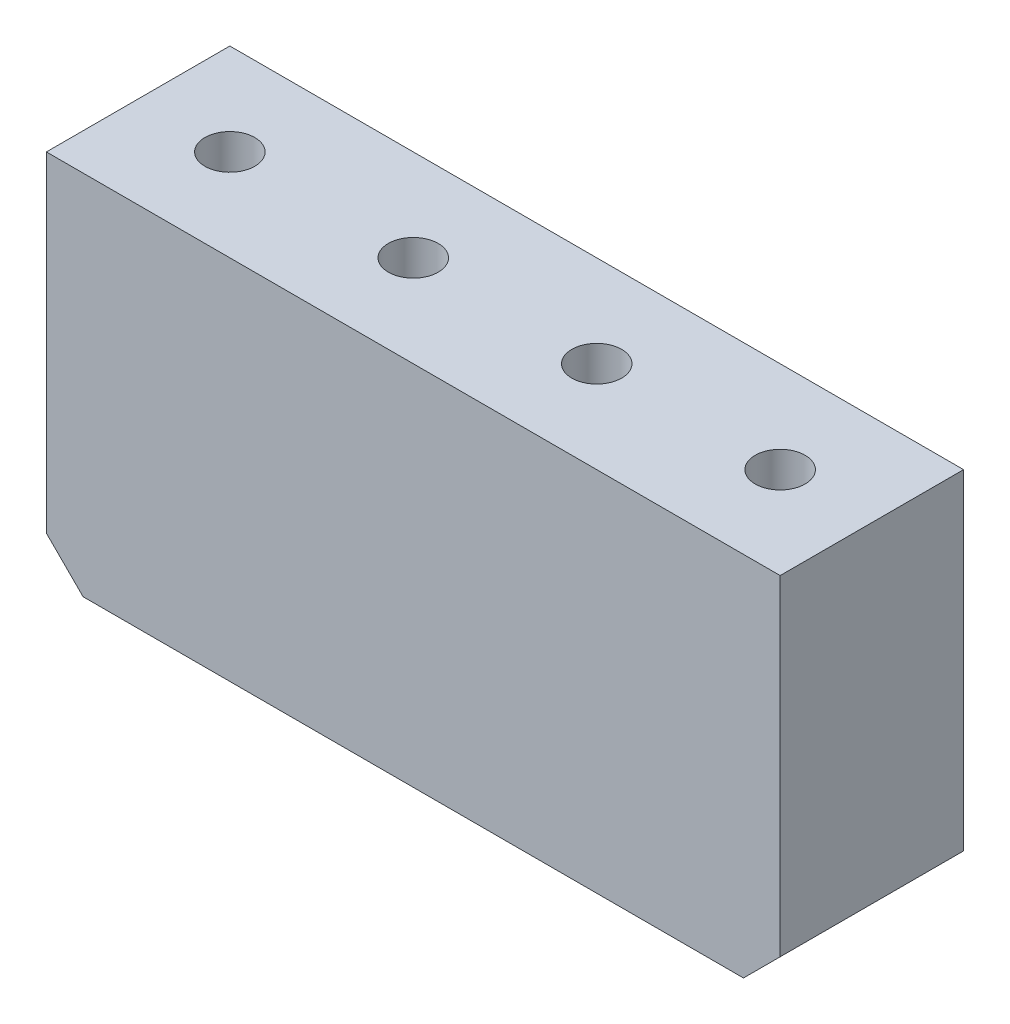
from build123d import *

# Parameters (mm, degrees)
SKETCH1_W           = 100
SKETCH1_H           = 50
BOSS_EXTRUDE1_DEPTH = 25
M8_TAPPED_HOLE1_D   = 6.8
CHAMFER1_SIZE       = 5


with BuildPart() as part:
    # Sketch1 → Boss-Extrude1 (new body)
    with BuildSketch(Plane.XY):
        Rectangle(SKETCH1_W, SKETCH1_H)
    extrude(amount=BOSS_EXTRUDE1_DEPTH)

    # M8 Tapped Hole1 (through all)
    with Locations(Plane(origin=(0, 25, 0), x_dir=(1, 0, 0), z_dir=(0, 1, 0))):
        with Locations((-37.5, -12.5), (-12.5, -12.5), (12.5, -12.5), (37.5, -12.5)):
            Hole(M8_TAPPED_HOLE1_D / 2)

    # Chamfer1
    chamfer1_edges = [part.edges().sort_by_distance(p)[0] for p in [
        (-50, -25, 12.5),
        (50, -25, 12.5),
    ]]
    chamfer(chamfer1_edges, length=CHAMFER1_SIZE)


solid = part.part
